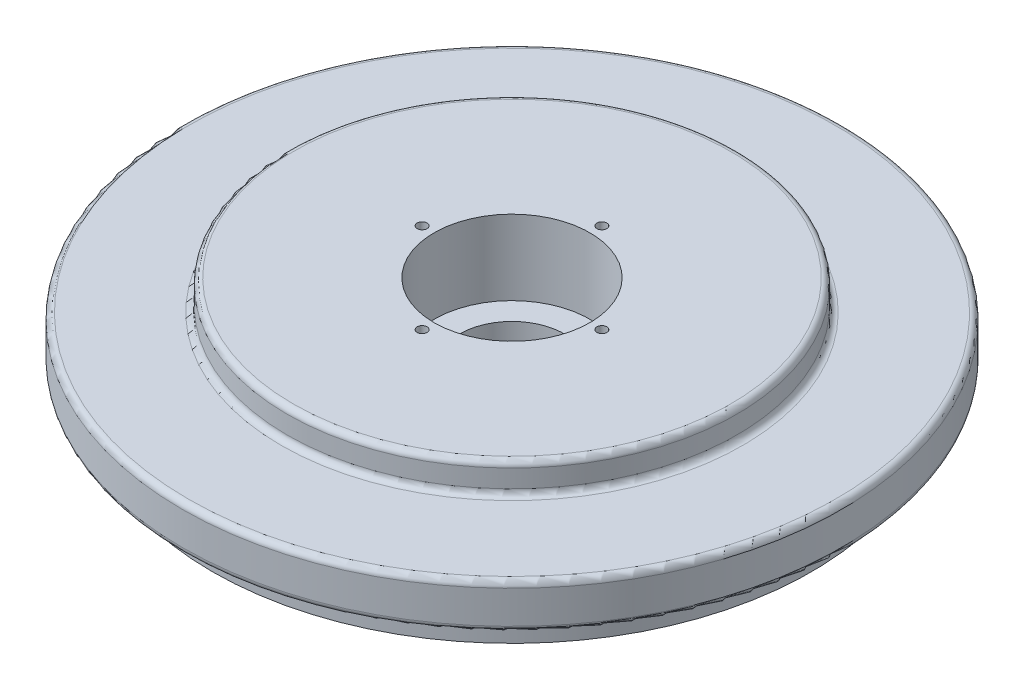
SolidWorks part; units mm, degrees
ref_plane "Front Plane" through (0, 0, 0) normal (0, 0, 1) x (1, 0, 0)
ref_plane "Top Plane" through (0, 0, 0) normal (0, 1, 0) x (1, 0, 0)
ref_plane "Right Plane" through (0, 0, 0) normal (1, 0, 0) x (0, 0, -1)
sketch "Sketch1" plane through (0, 0, 0) normal (0, 1, 0) x (1, 0, 0)
  circle A0 centre (0, 0) radius 100
  dimension "D1" = 200
extrude "Boss-Extrude1" add sketch "Sketch1" along normal blind 10
sketch "Sketch2" plane through (0, 10, 0) normal (0, 1, 0) x (1, 0, 0)
  circle A0 centre (0, 0) radius 110
  dimension "D1" = 220
extrude "Boss-Extrude2" add sketch "Sketch2" along normal blind 15
sketch "Sketch3" plane through (0, 25, 0) normal (0, 1, 0) x (1, 0, 0)
  circle A0 centre (0, 0) radius 75
  dimension "D1" = 150
extrude "Boss-Extrude3" add sketch "Sketch3" along normal blind 10
fillet "Fillet1" radius 2 2 edges at (0, 35, 75) (0, 25, 75)
sketch "Sketch4" plane through (0, 35, 0) normal (0, 1, 0) x (1, 0, 0)
  circle A0 centre (0, 0) radius 26
  dimension "D1" = 52
extrude "Cut-Extrude1" cut sketch "Sketch4" against normal blind 25
sketch "Sketch5" plane through (0, 10, 0) normal (0, 1, 0) x (1, 0, 0)
  circle A0 centre (0, 0) radius 17.5
  dimension "D1" = 35
extrude "Cut-Extrude2" cut sketch "Sketch5" against normal through all
sketch "Sketch6" plane through (0, 35, 0) normal (0, 1, 0) x (1, 0, 0)
  point P0 (0, 30)
  point P1 (30, 0)
  point P3 (-30, 0)
  point P5 (0, -30)
hole_wizard "M4 Tapped Hole1" positions "Sketch7" profile "Sketch8" tap size "M4" standard "GB"
sketch "Sketch7" plane through (0, 35, 0) normal (0, 1, 0) x (1, 0, 0)
  point P0 (0, 30)
sketch "Sketch8" plane through (0, 35, -30) normal (1, 0, 0) x (0, 0, 1)
  line L0 (0, 0) -> (0, 11.0914)
  line L1 (0, 11.0914) -> (1.65, 10.1)
  line L2 (1.65, 10.1) -> (1.65, 0)
  line L5 (1.65, 0) -> (0, 0)
  line L10 (0, 11.0914) -> (-1.65, 10.1) construction
  line L11 (0, -6.35) -> (0, 107.95) construction
  dimension "螺纹孔钻头直径" = 3.3
  dimension "螺纹孔钻头深度" = 10.1
  dimension "导头角度" = 118
cosmetic thread "Hole Thread1" parameters "D1"=8, "D2"=4
pattern_circular "CirPattern1" count 4 over 360 about axis through (0, 0, 0) along (0, 1, 0) of "M4 Tapped Hole1"
fillet "Fillet2" radius 2 2 edges at (0, 10, 110) (0, 25, 110)
